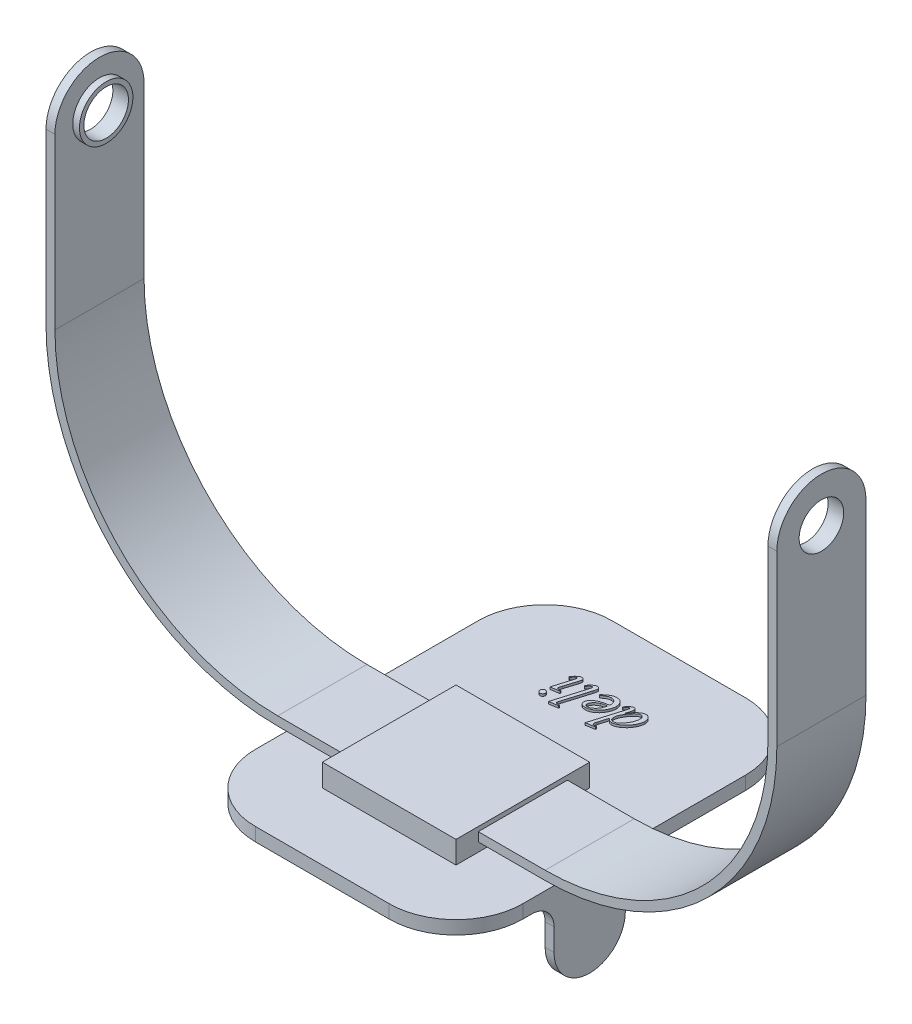
from build123d import *

# Parameters (mm, degrees)
BOSS_EXTRUDE1_DEPTH     = 3
SKETCH2_W               = 30
SKETCH2_H               = 5
BOSS_EXTRUDE2_DEPTH     = 15
BOSS_EXTRUDE3_DEPTH     = 10
BOSS_EXTRUDE4_START     = -82
SKETCH_4_2_R            = 10
BOSS_EXTRUDE4_DEPTH     = 2
BOSS_EXTRUDE5_START     = 80
SKETCH_4_2_2_R          = 10
BOSS_EXTRUDE5_DEPTH     = 2
CUT_EXTRUDE1_DEPTH      = 143.298981022
CUT_EXTRUDE1_DEPTH_BACK = 143.298981022
SKETCH5_R               = 5
SKETCH_6_2_R            = 6
SKETCH_6_2_R_2          = 5
BOSS_EXTRUDE6_DEPTH     = 1.5
BOSS_EXTRUDE7_START     = 158.5
SKETCH_6_2_2_R          = 6
SKETCH_6_2_2_R_2        = 5
BOSS_EXTRUDE7_DEPTH     = 1.5
BOSS_EXTRUDE8_START     = 30
BOSS_EXTRUDE8_DEPTH     = 2
BOSS_EXTRUDE9_START     = -28
BOSS_EXTRUDE9_DEPTH     = 2
BOSS_EXTRUDE10_START    = 28
SKETCH_8_2_R            = 5
BOSS_EXTRUDE10_DEPTH    = 2
BOSS_EXTRUDE11_START    = -26
SKETCH_8_2_2_R          = 5
BOSS_EXTRUDE11_DEPTH    = 2
FILLET1_R               = 5
SKETCH9_R               = 2.5
CUT_EXTRUDE4_DEPTH      = 27
BOSS_EXTRUDE12_DEPTH    = 0.5
BOSS_EXTRUDE12_2_DEPTH  = 0.5
BOSS_EXTRUDE12_3_DEPTH  = 0.5
BOSS_EXTRUDE12_4_DEPTH  = 0.5
BOSS_EXTRUDE12_5_DEPTH  = 0.5


with BuildPart() as part:
    # Sketch1 → Boss-Extrude1 (new body)
    with BuildSketch(Plane(origin=(0, 0, 0), x_dir=(1, 0, 0), z_dir=(0, 1, 0))):
        with BuildLine():
            Line((-15, 50), (15, 50))
            ThreePointArc((15, 50), (25.606601718, 45.606601718), (30, 35))
            Line((30, 35), (30, -15))
            ThreePointArc((30, -15), (25.606601718, -25.606601718), (15, -30))
            Line((15, -30), (-15, -30))
            ThreePointArc((-15, -30), (-25.606601718, -25.606601718), (-30, -15))
            Line((-30, -15), (-30, 35))
            ThreePointArc((-30, 35), (-25.606601718, 45.606601718), (-15, 50))
        make_face()
    extrude(amount=BOSS_EXTRUDE1_DEPTH)

    # Sketch2 → Boss-Extrude2 (add, symmetric)
    with BuildSketch(Plane.XY):
        with Locations((0, 5.5)):
            Rectangle(SKETCH2_W, SKETCH2_H)
    extrude(amount=BOSS_EXTRUDE2_DEPTH, both=True)

    # Sketch3 → Boss-Extrude3 (add, symmetric)
    with BuildSketch(Plane.XY):
        with BuildLine():
            Line((-15, 5), (-30, 5))
            ThreePointArc((-30, 5), (-66.769552622, 20.230447378), (-82, 57))
            Line((-82, 57), (-82, 95))
            Line((-82, 95), (-80, 95))
            Line((-80, 95), (-80, 57))
            ThreePointArc((-80, 57), (-65.355339059, 21.644660941), (-30, 7))
            Line((-30, 7), (-15, 7))
            Line((-15, 7), (-15, 5))
        make_face()
        with BuildLine():
            Line((15, 5), (15, 7))
            Line((15, 7), (30, 7))
            ThreePointArc((30, 7), (65.355339059, 21.644660941), (80, 57))
            Line((80, 57), (80, 95))
            Line((80, 95), (82, 95))
            Line((82, 95), (82, 57))
            ThreePointArc((82, 57), (66.769552622, 20.230447378), (30, 5))
            Line((30, 5), (15, 5))
        make_face()
    extrude(amount=BOSS_EXTRUDE3_DEPTH, both=True)

    # Sketch 4_2 → Boss-Extrude4 (add)
    with BuildSketch(Plane(origin=(0, 0, 0), x_dir=(0, 0, -1), z_dir=(1, 0, 0)).offset(BOSS_EXTRUDE4_START)):
        with Locations((0, 95)):
            Circle(SKETCH_4_2_R)
    extrude(amount=BOSS_EXTRUDE4_DEPTH)

    # Sketch 4_2 2 → Boss-Extrude5 (add)
    with BuildSketch(Plane(origin=(0, 0, 0), x_dir=(0, 0, -1), z_dir=(1, 0, 0)).offset(BOSS_EXTRUDE5_START)):
        with Locations((0, 95)):
            Circle(SKETCH_4_2_2_R)
    extrude(amount=BOSS_EXTRUDE5_DEPTH)

    # Sketch5 → Cut-Extrude1 (cut, two sides: drawn at the far end of the back side and taken through both)
    with BuildSketch(Plane(origin=(0, 0, 0), x_dir=(0, 0, -1), z_dir=(1, 0, 0)).offset(-CUT_EXTRUDE1_DEPTH_BACK)):
        with Locations((0, 95)):
            Circle(SKETCH5_R)
    extrude(amount=CUT_EXTRUDE1_DEPTH + CUT_EXTRUDE1_DEPTH_BACK, mode=Mode.SUBTRACT)

    # Sketch 6_2 → Boss-Extrude6 (add)
    with BuildSketch(Plane.ZY.offset(-80)):
        with Locations(Location((0, 95, 0), (0, 0, 90))):
            Circle(SKETCH_6_2_R)
        with Locations(Location((0, 95, 0), (0, 0, 180))):
            Circle(SKETCH_6_2_R_2, mode=Mode.SUBTRACT)
    extrude(amount=BOSS_EXTRUDE6_DEPTH)

    # Sketch 6_2 2 → Boss-Extrude7 (add)
    with BuildSketch(Plane.ZY.offset(-80).offset(BOSS_EXTRUDE7_START)):
        with Locations(Location((0, 95, 0), (0, 0, 90))):
            Circle(SKETCH_6_2_2_R)
        with Locations(Location((0, 95, 0), (0, 0, 180))):
            Circle(SKETCH_6_2_2_R_2, mode=Mode.SUBTRACT)
    extrude(amount=BOSS_EXTRUDE7_DEPTH)

    # Sketch 7_2 → Boss-Extrude8 (add)
    with BuildSketch(Plane(origin=(0, 0, 0), x_dir=(0, 0, -1), z_dir=(1, 0, 0)).offset(BOSS_EXTRUDE8_START)):
        with BuildLine():
            Line((-8, 0), (-8, -10))
            ThreePointArc((-8, -10), (0, -18), (8, -10))
            Line((8, -10), (8, 0))
            Line((8, 0), (-8, 0))
        make_face()
    extrude(amount=-BOSS_EXTRUDE8_DEPTH)

    # Sketch 7_2 2 → Boss-Extrude9 (add)
    with BuildSketch(Plane(origin=(0, 0, 0), x_dir=(0, 0, -1), z_dir=(1, 0, 0)).offset(BOSS_EXTRUDE9_START)):
        with BuildLine():
            Line((-8, 0), (-8, -10))
            ThreePointArc((-8, -10), (0, -18), (8, -10))
            Line((8, -10), (8, 0))
            Line((8, 0), (-8, 0))
        make_face()
    extrude(amount=-BOSS_EXTRUDE9_DEPTH)

    # Sketch 8_2 → Boss-Extrude10 (add)
    with BuildSketch(Plane(origin=(0, 0, 0), x_dir=(0, 0, -1), z_dir=(1, 0, 0)).offset(BOSS_EXTRUDE10_START)):
        with Locations(Location((0, -10, 0), (0, 0, 180))):
            Circle(SKETCH_8_2_R)
    extrude(amount=-BOSS_EXTRUDE10_DEPTH)

    # Sketch 8_2 2 → Boss-Extrude11 (add)
    with BuildSketch(Plane(origin=(0, 0, 0), x_dir=(0, 0, -1), z_dir=(1, 0, 0)).offset(BOSS_EXTRUDE11_START)):
        with Locations(Location((0, -10, 0), (0, 0, 180))):
            Circle(SKETCH_8_2_2_R)
    extrude(amount=-BOSS_EXTRUDE11_DEPTH)

    # Fillet1
    fillet1_edges = [part.edges().sort_by_distance(p)[0] for p in [
        (29, 0, -8),
        (29, 0, 8),
        (-29, 0, -8),
        (-29, 0, 8),
    ]]
    fillet(fillet1_edges, radius=FILLET1_R)

    # Sketch9 → Cut-Extrude4 (cut, symmetric)
    with BuildSketch(Plane(origin=(0, 0, 0), x_dir=(0, 0, -1), z_dir=(1, 0, 0))):
        with Locations((0, -10)):
            Circle(SKETCH9_R)
    extrude(amount=CUT_EXTRUDE4_DEPTH, both=True, mode=Mode.SUBTRACT)


with BuildPart() as body_2:
    # Sketch10 → Boss-Extrude12 (new body)
    with BuildSketch(Plane(origin=(0, 3, 0), x_dir=(1, 0, 0), z_dir=(0, 1, 0))):
        with BuildLine():
            add(Edge.make_bspline(
                [(-8.5, 27.333333333), (-8.541420185, 27.334812978), (-8.622373784, 27.337704865), (-8.736932892, 27.375906898), (-8.844424619, 27.428880052), (-8.936084754, 27.50835969), (-9.015564392, 27.600019826), (-9.068537547, 27.707511552), (-9.106739579, 27.82207066), (-9.109631467, 27.903024259), (-9.111111111, 27.944444444)],
                knots=[0, 0, 0, 0, 1.028598998, 2.010343287, 2.985271304, 4, 5.014728696, 5.989656713, 6.971401002, 8, 8, 8, 8], degree=3))
            add(Edge.make_bspline(
                [(-9.111111111, 27.944444444), (-9.108646384, 27.985182003), (-9.103842649, 28.064579182), (-9.069536389, 28.179728438), (-9.011227173, 28.284342378), (-8.932445255, 28.377966561), (-8.839646955, 28.456925089), (-8.73365261, 28.513832493), (-8.619904173, 28.550625499), (-8.540210548, 28.553902233), (-8.5, 28.555555556)],
                knots=[0, 0, 0, 0, 1.019615011, 1.987221587, 2.979692095, 3.998482675, 5.037687838, 6.010490816, 6.996164956, 8, 8, 8, 8], degree=3))
            add(Edge.make_bspline(
                [(-8.5, 28.555555556), (-8.459159441, 28.554062369), (-8.379341087, 28.551144101), (-8.265670403, 28.5128723), (-8.158837731, 28.458186193), (-8.067859872, 28.376584572), (-7.986258252, 28.285606713), (-7.931572144, 28.178774041), (-7.893300344, 28.065103357), (-7.890382076, 27.985285004), (-7.888888889, 27.944444444)],
                knots=[0, 0, 0, 0, 1.01730782, 1.988215549, 2.972847037, 4, 5.027152963, 6.011784451, 6.98269218, 8, 8, 8, 8], degree=3))
            add(Edge.make_bspline(
                [(-7.888888889, 27.944444444), (-7.890601218, 27.903104611), (-7.893940971, 27.822474766), (-7.928826842, 27.706673368), (-7.984962877, 27.600574964), (-8.063689528, 27.508193303), (-8.15536551, 27.429519959), (-8.262116951, 27.375062603), (-8.377174147, 27.338017063), (-8.458614823, 27.334911478), (-8.5, 27.333333333)],
                knots=[0, 0, 0, 0, 1.028140666, 2.005301341, 2.986502084, 4.000778629, 5.015055174, 5.976752111, 6.971859334, 8, 8, 8, 8], degree=3))
        make_face()
    extrude(amount=BOSS_EXTRUDE12_DEPTH)


with BuildPart() as body_3:
    # Sketch10 → Boss-Extrude12 2 (new body)
    with BuildSketch(Plane(origin=(0, 3, 0), x_dir=(1, 0, 0), z_dir=(0, 1, 0))):
        with BuildLine():
            Line((-8.585069444, 29.666666667), (-7.355902778, 33.802083333))
            add(Edge.make_bspline(
                [(-7.355902778, 33.802083333), (-7.336641834, 33.864396865), (-7.302367458, 33.975282264), (-7.266778457, 34.122567392), (-7.237721808, 34.226419245), (-7.232745277, 34.282905944), (-7.230902778, 34.303819444)],
                knots=[0, 0, 0, 0, 1.510565239, 2.688013749, 3.514253344, 4, 4, 4, 4], degree=3))
            add(Edge.make_bspline(
                [(-7.230902778, 34.303819444), (-7.232499568, 34.331792064), (-7.235560335, 34.385410663), (-7.279358856, 34.450998375), (-7.336872099, 34.499266152), (-7.38459256, 34.504418606), (-7.407986111, 34.506944444)],
                knots=[0, 0, 0, 0, 1.10317457, 2.11459187, 3.07573415, 4, 4, 4, 4], degree=3))
            add(Edge.make_bspline(
                [(-7.407986111, 34.506944444), (-7.438889271, 34.501321301), (-7.512022319, 34.488014001), (-7.57153679, 34.442784154), (-7.605902778, 34.416666667)],
                knots=[0, 0, 0, 0, 0.845121608, 2, 2, 2, 2], degree=3))
            add(Edge.make_bspline(
                [(-7.605902778, 34.416666667), (-7.659490786, 34.369589121), (-7.771584476, 34.271113809), (-7.928409803, 34.096916777), (-8.08743216, 33.896358008), (-8.187323661, 33.748978634), (-8.239583333, 33.671875)],
                knots=[0, 0, 0, 0, 0.871693875, 1.823381532, 2.861270808, 4, 4, 4, 4], degree=3))
            Line((-8.239583333, 33.671875), (-8.444444444, 33.805555556))
            add(Edge.make_bspline(
                [(-8.444444444, 33.805555556), (-8.380580766, 33.903281075), (-8.254738652, 34.095847277), (-8.042288813, 34.361978639), (-7.812479845, 34.602601835), (-7.644316334, 34.742828195), (-7.560763889, 34.8125)],
                knots=[0, 0, 0, 0, 1.040132415, 2.049560354, 3.030919369, 4, 4, 4, 4], degree=3))
            add(Edge.make_bspline(
                [(-7.560763889, 34.8125), (-7.500015929, 34.85773527), (-7.384375719, 34.943845423), (-7.20079883, 35.038480527), (-7.020527173, 35.098874143), (-6.90030187, 35.107115508), (-6.842013889, 35.111111111)],
                knots=[0, 0, 0, 0, 1.145591956, 2.180756243, 3.117988943, 4, 4, 4, 4], degree=3))
            add(Edge.make_bspline(
                [(-6.842013889, 35.111111111), (-6.806003893, 35.10940655), (-6.736576224, 35.106120136), (-6.636409075, 35.081738802), (-6.547396613, 35.037883132), (-6.470732424, 34.978241396), (-6.406982687, 34.907007436), (-6.362129247, 34.824215594), (-6.332148703, 34.733502142), (-6.329488644, 34.669805846), (-6.328125, 34.637152778)],
                knots=[0, 0, 0, 0, 1.105122397, 2.130688156, 3.139809048, 4.127749477, 5.097143713, 6.051441518, 7.001097123, 8, 8, 8, 8], degree=3))
            add(Edge.make_bspline(
                [(-6.328125, 34.637152778), (-6.330771912, 34.594231017), (-6.336859573, 34.495514801), (-6.369586849, 34.32975544), (-6.419979127, 34.127010951), (-6.465051562, 33.980683792), (-6.489583333, 33.901041667)],
                knots=[0, 0, 0, 0, 0.682294175, 1.56921566, 2.676986339, 4, 4, 4, 4], degree=3))
            Line((-6.489583333, 33.901041667), (-7.324652778, 31.222222222))
            add(Edge.make_bspline(
                [(-7.324652778, 31.222222222), (-7.339215054, 31.173059431), (-7.366939427, 31.07946091), (-7.404960277, 30.945731883), (-7.438456834, 30.826788212), (-7.464132617, 30.721795974), (-7.486019038, 30.631820439), (-7.499266075, 30.555734031), (-7.5090628, 30.494439571), (-7.511218086, 30.458356587), (-7.512152778, 30.442708333)],
                knots=[0, 0, 0, 0, 1.532168456, 2.917017096, 4.154648942, 5.224165243, 6.147037692, 6.920406562, 7.531808337, 8, 8, 8, 8], degree=3))
            add(Edge.make_bspline(
                [(-7.512152778, 30.442708333), (-7.511384228, 30.422874614), (-7.509882235, 30.384113149), (-7.491207849, 30.329294302), (-7.463127777, 30.279069294), (-7.422918657, 30.23627543), (-7.373743693, 30.200506521), (-7.314660272, 30.176777718), (-7.248551163, 30.160558141), (-7.201496508, 30.158864708), (-7.177083333, 30.157986111)],
                knots=[0, 0, 0, 0, 0.960320695, 1.876775426, 2.784115297, 3.739891537, 4.708011502, 5.716578817, 6.815301896, 8, 8, 8, 8], degree=3))
            add(Edge.make_bspline(
                [(-7.177083333, 30.157986111), (-7.150439511, 30.158808106), (-7.085964861, 30.160797228), (-6.972545176, 30.174750906), (-6.826226464, 30.195604448), (-6.717570824, 30.212795159), (-6.657986111, 30.222222222)],
                knots=[0, 0, 0, 0, 0.610863574, 1.478211924, 2.617098769, 4, 4, 4, 4], degree=3))
            Line((-6.657986111, 30.222222222), (-6.657986111, 30))
            Line((-6.657986111, 30), (-8.585069444, 29.666666667))
        make_face()
    extrude(amount=BOSS_EXTRUDE12_2_DEPTH)


with BuildPart() as body_4:
    # Sketch10 → Boss-Extrude12 3 (new body)
    with BuildSketch(Plane(origin=(0, 3, 0), x_dir=(1, 0, 0), z_dir=(0, 1, 0))):
        with BuildLine():
            Line((-5.918402778, 26.666666667), (-3.845486111, 33.645833333))
            add(Edge.make_bspline(
                [(-3.845486111, 33.645833333), (-3.833861782, 33.686907898), (-3.811608596, 33.765539522), (-3.780998638, 33.87666148), (-3.753680465, 33.975311461), (-3.734105637, 34.06140897), (-3.715343781, 34.135063714), (-3.70399099, 34.195999289), (-3.695502075, 34.244560262), (-3.694765106, 34.27254557), (-3.694444444, 34.284722222)],
                knots=[0, 0, 0, 0, 1.557950218, 2.982482127, 4.206953031, 5.292990824, 6.204869726, 6.979465914, 7.555956673, 8, 8, 8, 8], degree=3))
            add(Edge.make_bspline(
                [(-3.694444444, 34.284722222), (-3.696747268, 34.312124756), (-3.701293522, 34.366223076), (-3.748623623, 34.433229722), (-3.8132144, 34.482632309), (-3.866076892, 34.487274934), (-3.892361111, 34.489583333)],
                knots=[0, 0, 0, 0, 1.025489341, 2.024529968, 3.017759354, 4, 4, 4, 4], degree=3))
            add(Edge.make_bspline(
                [(-3.892361111, 34.489583333), (-3.932779005, 34.484248977), (-4.022520172, 34.472404933), (-4.09649497, 34.419630646), (-4.137152778, 34.390625)],
                knots=[0, 0, 0, 0, 0.900765954, 2, 2, 2, 2], degree=3))
            add(Edge.make_bspline(
                [(-4.137152778, 34.390625), (-4.190882826, 34.346041128), (-4.304544913, 34.251727124), (-4.463137323, 34.076831543), (-4.630239681, 33.873633443), (-4.734982313, 33.720801181), (-4.789930556, 33.640625)],
                knots=[0, 0, 0, 0, 0.838448543, 1.773678133, 2.832066056, 4, 4, 4, 4], degree=3))
            Line((-4.789930556, 33.640625), (-5.012152778, 33.819444444))
            add(Edge.make_bspline(
                [(-5.012152778, 33.819444444), (-4.966374089, 33.881763763), (-4.87746311, 34.002799813), (-4.739435572, 34.172525292), (-4.606549827, 34.329003896), (-4.475897574, 34.470599514), (-4.347390274, 34.596944352), (-4.222935406, 34.710824247), (-4.099526874, 34.808342595), (-4.015954375, 34.865045329), (-3.975694444, 34.892361111)],
                knots=[0, 0, 0, 0, 1.237412522, 2.403292069, 3.50032817, 4.522768916, 5.485533148, 6.38395291, 7.221490987, 8, 8, 8, 8], degree=3))
            add(Edge.make_bspline(
                [(-3.975694444, 34.892361111), (-3.919115386, 34.925562868), (-3.810117895, 34.989524841), (-3.641320815, 35.05978944), (-3.475454595, 35.102137894), (-3.365964105, 35.10816707), (-3.3125, 35.111111111)],
                knots=[0, 0, 0, 0, 1.112232707, 2.142675722, 3.093070267, 4, 4, 4, 4], degree=3))
            add(Edge.make_bspline(
                [(-3.3125, 35.111111111), (-3.276409209, 35.109719652), (-3.205967288, 35.107003804), (-3.105361253, 35.077600481), (-3.013576852, 35.032500215), (-2.934166202, 34.969533008), (-2.869143099, 34.896352575), (-2.820093084, 34.815524926), (-2.788995971, 34.72849685), (-2.786141632, 34.667490239), (-2.784722222, 34.637152778)],
                knots=[0, 0, 0, 0, 1.098796497, 2.144628464, 3.171642199, 4.203506084, 5.217216168, 6.144259147, 7.077174325, 8, 8, 8, 8], degree=3))
            add(Edge.make_bspline(
                [(-2.784722222, 34.637152778), (-2.785640561, 34.616880769), (-2.78766688, 34.572150475), (-2.796879424, 34.497897174), (-2.813344387, 34.410137743), (-2.833081455, 34.307147518), (-2.86462809, 34.191698432), (-2.896536972, 34.060348313), (-2.93642061, 33.915607505), (-2.966797255, 33.814750444), (-2.982638889, 33.762152778)],
                knots=[0, 0, 0, 0, 0.54157402, 1.194985938, 1.995025139, 2.925138508, 3.99297548, 5.188202046, 6.533627604, 8, 8, 8, 8], degree=3))
            Line((-2.982638889, 33.762152778), (-4.65625, 28.222222222))
            add(Edge.make_bspline(
                [(-4.65625, 28.222222222), (-4.671213689, 28.171851415), (-4.699420561, 28.076901375), (-4.740506513, 27.943139826), (-4.772070085, 27.825674077), (-4.801437835, 27.726136505), (-4.821296141, 27.642968594), (-4.838086406, 27.576792098), (-4.846855826, 27.527386388), (-4.849635481, 27.5000121), (-4.850694444, 27.489583333)],
                knots=[0, 0, 0, 0, 1.662132792, 3.133155605, 4.425573519, 5.509286808, 6.414969554, 7.129803733, 7.668481851, 8, 8, 8, 8], degree=3))
            add(Edge.make_bspline(
                [(-4.850694444, 27.489583333), (-4.849515113, 27.467958678), (-4.847223044, 27.425930468), (-4.824331735, 27.366104065), (-4.789510124, 27.311689246), (-4.739324236, 27.263724428), (-4.674223424, 27.225252155), (-4.593365056, 27.20054455), (-4.499646441, 27.182392505), (-4.43182031, 27.181192337), (-4.395833333, 27.180555556)],
                knots=[0, 0, 0, 0, 0.837269546, 1.627260187, 2.45724371, 3.33234812, 4.300800159, 5.36796539, 6.603503304, 8, 8, 8, 8], degree=3))
            add(Edge.make_bspline(
                [(-4.395833333, 27.180555556), (-4.370365971, 27.181597106), (-4.314166503, 27.183895521), (-4.220780737, 27.190534828), (-4.111045318, 27.205588792), (-4.031825689, 27.216437406), (-3.989583333, 27.222222222)],
                knots=[0, 0, 0, 0, 0.748511941, 1.651760119, 2.747845874, 4, 4, 4, 4], degree=3))
            Line((-3.989583333, 27.222222222), (-3.989583333, 27))
            Line((-3.989583333, 27), (-5.918402778, 26.666666667))
        make_face()
    extrude(amount=BOSS_EXTRUDE12_3_DEPTH)


with BuildPart() as body_5:
    # Sketch10 → Boss-Extrude12 4 (new body)
    with BuildSketch(Plane(origin=(0, 3, 0), x_dir=(1, 0, 0), z_dir=(0, 1, 0))):
        with BuildLine():
            add(Edge.make_bspline(
                [(1.666666667, 32.777777778), (1.666666667, 32.863425926), (1.666666667, 33.018518519), (1.666666667, 33.173611111), (1.666666667, 33.243055556)],
                knots=[0, 0, 0, 0, 1.104477612, 2, 2, 2, 2], degree=3))
            add(Edge.make_bspline(
                [(1.666666667, 33.243055556), (1.662273788, 33.323925427), (1.65368835, 33.481977421), (1.587582227, 33.709676638), (1.475380481, 33.916486773), (1.322787826, 34.098925866), (1.140257096, 34.250528365), (0.935548724, 34.366184754), (0.708125933, 34.431097887), (0.55073583, 34.439937382), (0.470486111, 34.444444444)],
                knots=[0, 0, 0, 0, 1.028786976, 2.010660195, 2.989902786, 4.005140265, 5.020377745, 5.996676742, 6.978549961, 8, 8, 8, 8], degree=3))
            add(Edge.make_bspline(
                [(0.470486111, 34.444444444), (0.404975823, 34.442417683), (0.273794292, 34.438359182), (0.079269388, 34.406212361), (-0.111401748, 34.35347403), (-0.268667348, 34.292659261), (-0.397543856, 34.227241154), (-0.506565498, 34.16668076), (-0.626219672, 34.09336052), (-0.757168987, 34.00783114), (-0.898899176, 33.908462178), (-1.05315088, 33.79776046), (-1.218579551, 33.674493048), (-1.330662044, 33.585935957), (-1.388888889, 33.539930556)],
                knots=[0, 0, 0, 0, 1.116743268, 2.236230327, 3.351926566, 4.486321476, 5.104204958, 5.815442257, 6.612617513, 7.49674141, 8.482286415, 9.564122796, 10.734561995, 12, 12, 12, 12], degree=3))
            Line((-1.388888889, 33.539930556), (-1.503472222, 33.710069444))
            add(Edge.make_bspline(
                [(-1.503472222, 33.710069444), (-1.394932978, 33.82091398), (-1.185657993, 34.034633807), (-0.859825072, 34.320333545), (-0.539124956, 34.56406089), (-0.219489298, 34.761318646), (0.09503685, 34.918725668), (0.407461689, 35.02909984), (0.716432774, 35.096743733), (0.921558629, 35.106370547), (1.022569444, 35.111111111)],
                knots=[0, 0, 0, 0, 1.254515299, 2.418836342, 3.502049071, 4.508850131, 5.453022715, 6.341327085, 7.183214109, 8, 8, 8, 8], degree=3))
            add(Edge.make_bspline(
                [(1.022569444, 35.111111111), (1.088599467, 35.109313951), (1.217073246, 35.105817241), (1.403673804, 35.082534509), (1.576794688, 35.038217638), (1.737518051, 34.979177206), (1.887311183, 34.904679149), (2.022583591, 34.81012195), (2.145939979, 34.699586978), (2.254046628, 34.572589159), (2.349147943, 34.436268471), (2.436117994, 34.297135583), (2.506590432, 34.153106693), (2.564771187, 34.005656554), (2.609593721, 33.854541278), (2.642941709, 33.700262705), (2.662358273, 33.542160604), (2.665218001, 33.435815949), (2.666666667, 33.381944444)],
                knots=[0, 0, 0, 0, 1.184036485, 2.303764805, 3.363266793, 4.380991813, 5.369413586, 6.353796734, 7.3309895, 8.331536943, 9.336325947, 10.30976536, 11.270344888, 12.206803224, 13.148992693, 14.093293866, 15.034111047, 16, 16, 16, 16], degree=3))
            add(Edge.make_bspline(
                [(2.666666667, 33.381944444), (2.664615037, 33.308991972), (2.660486325, 33.162181939), (2.638761175, 32.94068756), (2.595178814, 32.71915618), (2.540740155, 32.495284737), (2.465950739, 32.271839578), (2.380466489, 32.044492729), (2.27313442, 31.818563542), (2.154463458, 31.592306838), (2.024345078, 31.372086179), (1.882423282, 31.163032209), (1.73475597, 30.965526234), (1.57650788, 30.782152265), (1.412586091, 30.609855197), (1.238031768, 30.451499589), (1.055558243, 30.3059873), (0.867404702, 30.171853095), (0.67255805, 30.054913429), (0.477500605, 29.949930368), (0.279966846, 29.862882255), (0.08116093, 29.790869879), (-0.119817135, 29.7358492), (-0.321553705, 29.695060431), (-0.524951568, 29.67251628), (-0.66082886, 29.66862416), (-0.729166667, 29.666666667)],
                knots=[0, 0, 0, 0, 0.95300258, 1.917828616, 2.902054499, 3.899194863, 4.924492056, 5.977138973, 7.069252795, 8.188231816, 9.313268635, 10.407446328, 11.486670761, 12.531830279, 13.568787606, 14.590625095, 15.606857598, 16.615445646, 17.605688484, 18.572613802, 19.506485374, 20.422074245, 21.331497674, 22.225241579, 23.107407168, 24, 24, 24, 24], degree=3))
            add(Edge.make_bspline(
                [(-0.729166667, 29.666666667), (-0.821475353, 29.668975443), (-0.994834879, 29.673311421), (-1.235366207, 29.722786048), (-1.44134144, 29.79826344), (-1.604629755, 29.912360256), (-1.732168314, 30.045166565), (-1.821388861, 30.193342595), (-1.880187889, 30.352782834), (-1.885955772, 30.464183325), (-1.888888889, 30.520833333)],
                knots=[0, 0, 0, 0, 1.369651887, 2.57226283, 3.634333396, 4.605264403, 5.505640026, 6.350801257, 7.161340106, 8, 8, 8, 8], degree=3))
            add(Edge.make_bspline(
                [(-1.888888889, 30.520833333), (-1.884768766, 30.602403129), (-1.876494583, 30.766214578), (-1.800888933, 31.006485185), (-1.686981519, 31.242768238), (-1.577452117, 31.38487461), (-1.520833333, 31.458333333)],
                knots=[0, 0, 0, 0, 0.950697565, 1.90922565, 2.919220784, 4, 4, 4, 4], degree=3))
            add(Edge.make_bspline(
                [(-1.520833333, 31.458333333), (-1.478743522, 31.506477536), (-1.393527856, 31.603951015), (-1.249851971, 31.739603848), (-1.091581212, 31.867817084), (-0.919149842, 31.989291167), (-0.733477366, 32.104359891), (-0.532314879, 32.209301205), (-0.318777645, 32.311400146), (-0.168791437, 32.37069089), (-0.092013889, 32.401041667)],
                knots=[0, 0, 0, 0, 0.886584713, 1.794992782, 2.736453474, 3.709679608, 4.718787432, 5.763685496, 6.855236437, 8, 8, 8, 8], degree=3))
            add(Edge.make_bspline(
                [(-0.092013889, 32.401041667), (-0.037202431, 32.421197678), (0.076198824, 32.462899123), (0.256423821, 32.518337752), (0.452277721, 32.56999156), (0.664246926, 32.618357505), (0.892317582, 32.663725761), (1.136326615, 32.704047393), (1.395810403, 32.745633401), (1.574563507, 32.766847262), (1.666666667, 32.777777778)],
                knots=[0, 0, 0, 0, 0.777323672, 1.608230904, 2.508920293, 3.473223157, 4.502109922, 5.603973043, 6.765438753, 8, 8, 8, 8], degree=3))
        make_face()
        with BuildLine():
            add(Edge.make_bspline(
                [(1.626736111, 32.444444444), (1.494547348, 32.426875818), (1.241724828, 32.393274289), (0.882877495, 32.321005573), (0.561752499, 32.231066902), (0.365737132, 32.152111482), (0.272569444, 32.114583333)],
                knots=[0, 0, 0, 0, 1.143937487, 2.187880059, 3.138684756, 4, 4, 4, 4], degree=3))
            add(Edge.make_bspline(
                [(0.272569444, 32.114583333), (0.163233862, 32.061708206), (-0.046171104, 31.960439124), (-0.330406745, 31.78104857), (-0.570494354, 31.584673411), (-0.7654438, 31.374481015), (-0.917073264, 31.159926351), (-1.02583292, 30.948463975), (-1.099077491, 30.742039192), (-1.1071836, 30.603555447), (-1.111111111, 30.536458333)],
                knots=[0, 0, 0, 0, 1.320970071, 2.52998782, 3.648429459, 4.686820474, 5.640802702, 6.49706334, 7.271808317, 8, 8, 8, 8], degree=3))
            add(Edge.make_bspline(
                [(-1.111111111, 30.536458333), (-1.11000903, 30.497989209), (-1.107884604, 30.423834209), (-1.075567315, 30.31984745), (-1.031487206, 30.224763176), (-0.964003196, 30.144351482), (-0.879614412, 30.079770817), (-0.779520523, 30.031449949), (-0.663474354, 30.00411748), (-0.58116271, 30.001412206), (-0.538194444, 30)],
                knots=[0, 0, 0, 0, 1.035937183, 1.99692409, 2.920873487, 3.854712028, 4.803255543, 5.776275044, 6.839172688, 8, 8, 8, 8], degree=3))
            add(Edge.make_bspline(
                [(-0.538194444, 30), (-0.490056688, 30.00238663), (-0.391886019, 30.007253849), (-0.243412132, 30.035478551), (-0.093562826, 30.085268519), (0.058106057, 30.153607545), (0.211205371, 30.241272967), (0.366738496, 30.348188079), (0.523405533, 30.475391612), (0.68318547, 30.618652361), (0.839585901, 30.780178104), (0.983365545, 30.964771369), (1.118998012, 31.165488584), (1.242346207, 31.385949979), (1.354757997, 31.624032761), (1.457240664, 31.88030214), (1.549655756, 32.155003562), (1.600607643, 32.346330641), (1.626736111, 32.444444444)],
                knots=[0, 0, 0, 0, 0.663850529, 1.353836474, 2.075337692, 2.835913239, 3.643325243, 4.50406966, 5.434726298, 6.423181615, 7.461345315, 8.529063653, 9.644186456, 10.797932208, 12.007604354, 13.271207642, 14.600657047, 16, 16, 16, 16], degree=3))
        make_face(mode=Mode.SUBTRACT)
    extrude(amount=BOSS_EXTRUDE12_4_DEPTH)


with BuildPart() as body_6:
    # Sketch10 → Boss-Extrude12 5 (new body)
    with BuildSketch(Plane(origin=(0, 3, 0), x_dir=(1, 0, 0), z_dir=(0, 1, 0))):
        with BuildLine():
            Line((2.321180556, 26.666666667), (4.40625, 33.663194444))
            add(Edge.make_bspline(
                [(4.40625, 33.663194444), (4.419730368, 33.708283917), (4.445597994, 33.7948066), (4.479764991, 33.918823274), (4.509742927, 34.030966632), (4.534622245, 34.130308917), (4.550962819, 34.218152783), (4.566506047, 34.292386606), (4.572948872, 34.355230155), (4.575329137, 34.392935075), (4.576388889, 34.409722222)],
                knots=[0, 0, 0, 0, 1.47202792, 2.824690546, 4.023365925, 5.103410762, 6.0264145, 6.81813934, 7.47380691, 8, 8, 8, 8], degree=3))
            add(Edge.make_bspline(
                [(4.576388889, 34.409722222), (4.573624869, 34.426502513), (4.567642999, 34.462818278), (4.530633535, 34.506209595), (4.487324186, 34.543787116), (4.450822598, 34.548279995), (4.434027778, 34.550347222)],
                knots=[0, 0, 0, 0, 0.925808176, 2.003626301, 3.081444425, 4, 4, 4, 4], degree=3))
            add(Edge.make_bspline(
                [(4.434027778, 34.550347222), (4.407997115, 34.546688263), (4.34694947, 34.538107197), (4.295268976, 34.503961183), (4.265625, 34.484375)],
                knots=[0, 0, 0, 0, 0.852798269, 2, 2, 2, 2], degree=3))
            add(Edge.make_bspline(
                [(4.265625, 34.484375), (4.24858878, 34.471953685), (4.210679665, 34.444313688), (4.153890816, 34.390671147), (4.087836165, 34.32474854), (4.014059159, 34.245109516), (3.931331372, 34.152846818), (3.844259497, 34.044607967), (3.746181773, 33.924934609), (3.67924277, 33.839824805), (3.644097222, 33.795138889)],
                knots=[0, 0, 0, 0, 0.543367614, 1.209105392, 2.01130862, 2.951264364, 4.008693175, 5.207080678, 6.533610078, 8, 8, 8, 8], degree=3))
            Line((3.644097222, 33.795138889), (3.444444444, 33.918402778))
            add(Edge.make_bspline(
                [(3.444444444, 33.918402778), (3.50650579, 34.008824361), (3.625906505, 34.182787746), (3.81417697, 34.421825234), (4.006361369, 34.625713207), (4.195589791, 34.798782912), (4.384518223, 34.935788548), (4.569375084, 35.034229797), (4.748628165, 35.099235642), (4.868161588, 35.107268253), (4.925347222, 35.111111111)],
                knots=[0, 0, 0, 0, 1.337737896, 2.573693174, 3.707410459, 4.752177563, 5.698417181, 6.544759625, 7.30380272, 8, 8, 8, 8], degree=3))
            add(Edge.make_bspline(
                [(4.925347222, 35.111111111), (4.954523987, 35.109621225), (5.011242892, 35.106724924), (5.092232718, 35.078503888), (5.166304536, 35.035069678), (5.230502741, 34.972251262), (5.28685458, 34.897281585), (5.325048713, 34.804204079), (5.349811265, 34.698651815), (5.351533167, 34.622842292), (5.352430556, 34.583333333)],
                knots=[0, 0, 0, 0, 0.917494356, 1.783586241, 2.676029852, 3.605975778, 4.599362991, 5.613508553, 6.75625399, 8, 8, 8, 8], degree=3))
            add(Edge.make_bspline(
                [(5.352430556, 34.583333333), (5.350167599, 34.524191814), (5.345235699, 34.39529849), (5.309360721, 34.189286043), (5.252844116, 33.955486638), (5.203426293, 33.792006701), (5.177083333, 33.704861111)],
                knots=[0, 0, 0, 0, 0.789415496, 1.720456083, 2.784852739, 4, 4, 4, 4], degree=3))
            Line((5.177083333, 33.704861111), (4.951388889, 32.928819444))
            add(Edge.make_bspline(
                [(4.951388889, 32.928819444), (5.026190506, 33.03502627), (5.171237134, 33.24097024), (5.389220317, 33.535473322), (5.605123547, 33.802735552), (5.813824429, 34.045612531), (6.017934037, 34.262700629), (6.217016659, 34.453625175), (6.411287867, 34.620262876), (6.54391879, 34.716106475), (6.607638889, 34.762152778)],
                knots=[0, 0, 0, 0, 1.255519303, 2.434557542, 3.54041581, 4.575388153, 5.528932044, 6.419014521, 7.240444464, 8, 8, 8, 8], degree=3))
            add(Edge.make_bspline(
                [(6.607638889, 34.762152778), (6.690818293, 34.815458351), (6.850691528, 34.917913213), (7.102178013, 35.027620578), (7.34879204, 35.096448823), (7.512327987, 35.106307358), (7.592013889, 35.111111111)],
                knots=[0, 0, 0, 0, 1.117706751, 2.148264892, 3.097707962, 4, 4, 4, 4], degree=3))
            add(Edge.make_bspline(
                [(7.592013889, 35.111111111), (7.631415154, 35.109509006), (7.708856745, 35.106360132), (7.823344768, 35.089368356), (7.933172962, 35.057346067), (8.039762695, 35.013819922), (8.142521227, 34.957581202), (8.242463977, 34.890184987), (8.335275427, 34.807074625), (8.426417996, 34.715814131), (8.508491993, 34.612804239), (8.580960699, 34.500099246), (8.641211989, 34.378135146), (8.692162329, 34.247670662), (8.72977852, 34.107786794), (8.757287308, 33.959767285), (8.775453131, 33.803110752), (8.776990489, 33.695654112), (8.777777778, 33.640625)],
                knots=[0, 0, 0, 0, 0.89781008, 1.764609361, 2.628196033, 3.497097134, 4.381749991, 5.292050271, 6.235616572, 7.21424873, 8.226990357, 9.228780307, 10.260302398, 11.320149793, 12.413718106, 13.553719321, 14.747246774, 16, 16, 16, 16], degree=3))
            add(Edge.make_bspline(
                [(8.777777778, 33.640625), (8.776183534, 33.567046596), (8.772958796, 33.418216699), (8.743811375, 33.193505122), (8.696458087, 32.96569968), (8.631697514, 32.734415317), (8.550062032, 32.498481642), (8.447170399, 32.260145673), (8.326093902, 32.017951115), (8.191118804, 31.77357795), (8.038964456, 31.533770254), (7.874230085, 31.303207091), (7.698714525, 31.083512108), (7.510276163, 30.875928635), (7.30921297, 30.680460855), (7.096987555, 30.496290687), (6.873923273, 30.322519252), (6.716548468, 30.217774401), (6.637152778, 30.164930556)],
                knots=[0, 0, 0, 0, 0.833473324, 1.685898891, 2.563014491, 3.468309917, 4.405717278, 5.389918874, 6.407567712, 7.473169035, 8.552005657, 9.623823853, 10.682786103, 11.736619191, 12.798582258, 13.858417243, 14.919570116, 16, 16, 16, 16], degree=3))
            add(Edge.make_bspline(
                [(6.637152778, 30.164930556), (6.575044962, 30.125510608), (6.453226802, 30.048192394), (6.268614334, 29.946123818), (6.08751207, 29.860657572), (5.910622813, 29.790663201), (5.73823161, 29.7340494), (5.568262944, 29.696779417), (5.403056032, 29.669902881), (5.293506524, 29.667734166), (5.239583333, 29.666666667)],
                knots=[0, 0, 0, 0, 1.173471214, 2.301644333, 3.363125489, 4.366135457, 5.335563204, 6.253916626, 7.140531177, 8, 8, 8, 8], degree=3))
            add(Edge.make_bspline(
                [(5.239583333, 29.666666667), (5.185636996, 29.668080156), (5.081021962, 29.670821255), (4.929601295, 29.699347452), (4.790083614, 29.746326357), (4.659272665, 29.811619286), (4.537554117, 29.902169377), (4.417628772, 30.013897861), (4.299313434, 30.150772884), (4.225996373, 30.253403639), (4.1875, 30.307291667)],
                knots=[0, 0, 0, 0, 1.001322896, 1.941807993, 2.849584095, 3.729491574, 4.645633284, 5.65746377, 6.770011415, 8, 8, 8, 8], degree=3))
            Line((4.1875, 30.307291667), (3.598958333, 28.288194444))
            add(Edge.make_bspline(
                [(3.598958333, 28.288194444), (3.587175166, 28.248902517), (3.564864882, 28.174507066), (3.53638435, 28.067975793), (3.508072485, 27.974544727), (3.490717042, 27.916094675), (3.482638889, 27.888888889)],
                knots=[0, 0, 0, 0, 1.183476206, 2.240797312, 3.18117281, 4, 4, 4, 4], degree=3))
            add(Edge.make_bspline(
                [(3.482638889, 27.888888889), (3.471855347, 27.850794748), (3.451394563, 27.778514605), (3.427975204, 27.674375393), (3.41583707, 27.58013763), (3.412856306, 27.520857731), (3.411458333, 27.493055556)],
                knots=[0, 0, 0, 0, 1.177724321, 2.234624048, 3.172041568, 4, 4, 4, 4], degree=3))
            add(Edge.make_bspline(
                [(3.411458333, 27.493055556), (3.415116978, 27.45263745), (3.422315302, 27.373115501), (3.474391992, 27.312696392), (3.5, 27.282986111)],
                knots=[0, 0, 0, 0, 1.016527024, 2, 2, 2, 2], degree=3))
            add(Edge.make_bspline(
                [(3.5, 27.282986111), (3.521388918, 27.266908716), (3.564432465, 27.234554198), (3.641549652, 27.20418977), (3.725842229, 27.184432104), (3.785174371, 27.181880191), (3.815972222, 27.180555556)],
                knots=[0, 0, 0, 0, 0.944220076, 1.900170045, 2.910030047, 4, 4, 4, 4], degree=3))
            add(Edge.make_bspline(
                [(3.815972222, 27.180555556), (3.842016542, 27.18162783), (3.901675647, 27.184084063), (4.002001365, 27.190472692), (4.123856756, 27.205971366), (4.212379022, 27.216505663), (4.260416667, 27.222222222)],
                knots=[0, 0, 0, 0, 0.700431615, 1.604462082, 2.700033272, 4, 4, 4, 4], degree=3))
            Line((4.260416667, 27.222222222), (4.260416667, 27))
            Line((4.260416667, 27), (2.321180556, 26.666666667))
        make_face()
        with BuildLine():
            add(Edge.make_bspline(
                [(4.465277778, 30.829861111), (4.467580906, 30.770542009), (4.472030107, 30.655948923), (4.516741015, 30.492722447), (4.590520654, 30.34780109), (4.692011841, 30.223722196), (4.816007744, 30.124315743), (4.958223774, 30.051690758), (5.116545883, 30.006978047), (5.227712904, 30.002365456), (5.284722222, 30)],
                knots=[0, 0, 0, 0, 1.085355701, 2.096698267, 3.07403207, 4.0465757, 5.012443082, 5.966057455, 6.956941767, 8, 8, 8, 8], degree=3))
            add(Edge.make_bspline(
                [(5.284722222, 30), (5.351105357, 30.003782138), (5.486834426, 30.011515217), (5.688757793, 30.073581126), (5.893079832, 30.168608276), (6.097193735, 30.304462891), (6.303817088, 30.477223851), (6.51076651, 30.688481542), (6.721267694, 30.936243285), (6.927405148, 31.215567138), (7.123800484, 31.511077263), (7.296837171, 31.811281581), (7.446792114, 32.106996652), (7.565758374, 32.400749184), (7.661836645, 32.690225382), (7.727055377, 32.977509119), (7.769218731, 33.26148612), (7.774944774, 33.450089711), (7.777777778, 33.543402778)],
                knots=[0, 0, 0, 0, 0.686708664, 1.40406638, 2.171262037, 3.016090114, 3.935793475, 4.95758207, 6.076185345, 7.301759194, 8.552320215, 9.750437915, 10.890055641, 11.984568321, 13.031228611, 14.046451826, 15.03346713, 16, 16, 16, 16], degree=3))
            add(Edge.make_bspline(
                [(7.777777778, 33.543402778), (7.775331186, 33.612499864), (7.770699664, 33.74330415), (7.730553928, 33.926619667), (7.665404994, 34.085762636), (7.570009997, 34.214799615), (7.458091638, 34.316259194), (7.33437005, 34.391831378), (7.198063465, 34.437003002), (7.103335114, 34.441949503), (7.055555556, 34.444444444)],
                knots=[0, 0, 0, 0, 1.27985536, 2.422831077, 3.46128838, 4.444320009, 5.371158727, 6.247154979, 7.115891287, 8, 8, 8, 8], degree=3))
            add(Edge.make_bspline(
                [(7.055555556, 34.444444444), (6.997829788, 34.439852533), (6.876036877, 34.430164273), (6.690963549, 34.364580437), (6.500601881, 34.257767178), (6.300174634, 34.112086821), (6.091862455, 33.925773651), (5.874518871, 33.698129012), (5.649424706, 33.429057996), (5.420542059, 33.129043996), (5.20104963, 32.813989751), (5.006875857, 32.50014662), (4.840027069, 32.197238637), (4.704185543, 31.904538035), (4.598267672, 31.621408659), (4.523643786, 31.348926034), (4.475173452, 31.086203473), (4.468524506, 30.913965933), (4.465277778, 30.829861111)],
                knots=[0, 0, 0, 0, 0.590921355, 1.246757482, 1.989224418, 2.821334428, 3.778449888, 4.847101006, 6.041297706, 7.368669608, 8.709948649, 9.971196266, 11.14590201, 12.248831057, 13.272491231, 14.237061429, 15.1391445, 16, 16, 16, 16], degree=3))
        make_face(mode=Mode.SUBTRACT)
    extrude(amount=BOSS_EXTRUDE12_5_DEPTH)


solid = Compound([part.part, body_2.part, body_3.part, body_4.part, body_5.part, body_6.part])
